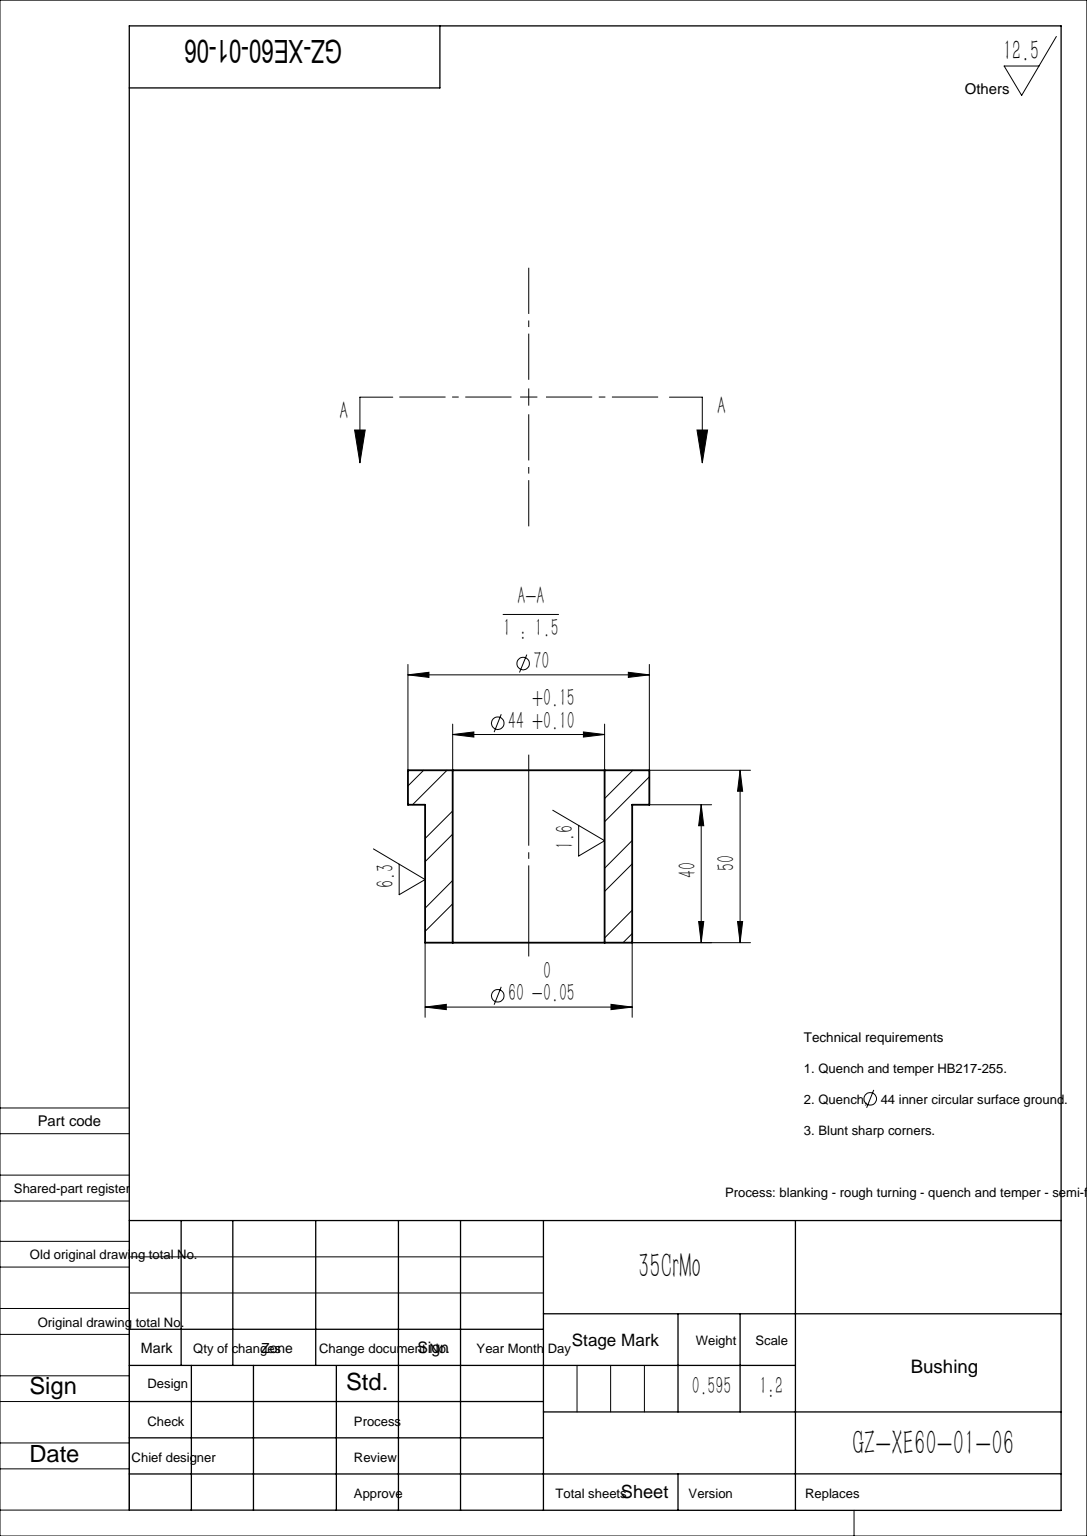
SolidWorks part; units mm, degrees
material "35CrMo"
ref_plane "Front Plane" through (0, 0, 0) normal (0, 0, 1) x (1, 0, 0)
ref_plane "Top Plane" through (0, 0, 0) normal (0, 1, 0) x (1, 0, 0)
ref_plane "Right Plane" through (0, 0, 0) normal (1, 0, 0) x (0, 0, -1)
sketch "Sketch1" plane through (0, 0, 0) normal (0, 0, 1) x (1, 0, 0)
  circle A0 centre (0, 0) radius 22
  circle A1 centre (0, 0) radius 30
  dimension "D1" = 60
  dimension "D2" = 44
extrude "Boss-Extrude1" add sketch "Sketch1" along normal blind 40
sketch "Sketch2" plane through (0, 0, 0) normal (0, 0, -1) x (-1, 0, 0)
  circle A0 centre (0, 0) radius 35
  circle A1 centre (0, 0) radius 22
  dimension "D1" = 70
extrude "Boss-Extrude2" add sketch "Sketch2" along normal blind 10
